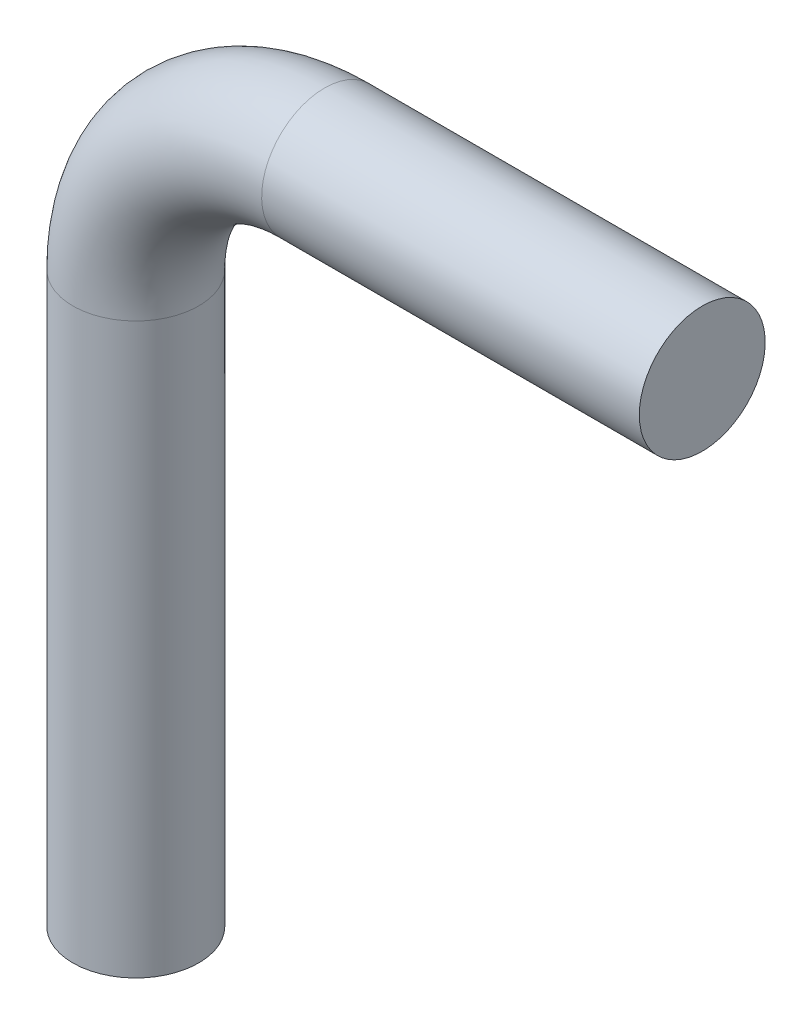
from build123d import *

# Parameters (mm, degrees)
SKETCH2_R = 3.175


with BuildPart() as part:
    # Sweep1: sweep along a path in Sketch1
    with BuildLine(Plane.XY) as sweep1_path:
        Line((0, 0), (0, 28.702))
        ThreePointArc((0, 28.702), (2.789807909, 35.437192091), (9.525, 38.227))
        Line((9.525, 38.227), (28.575, 38.227))
    # Sketch2 → Sweep1 (sweep)
    with BuildSketch(Plane(origin=(0, 0, 0), x_dir=(1, 0, 0), z_dir=(0, 1, 0))):
        Circle(SKETCH2_R)
    sweep(path=sweep1_path.line)


solid = part.part
